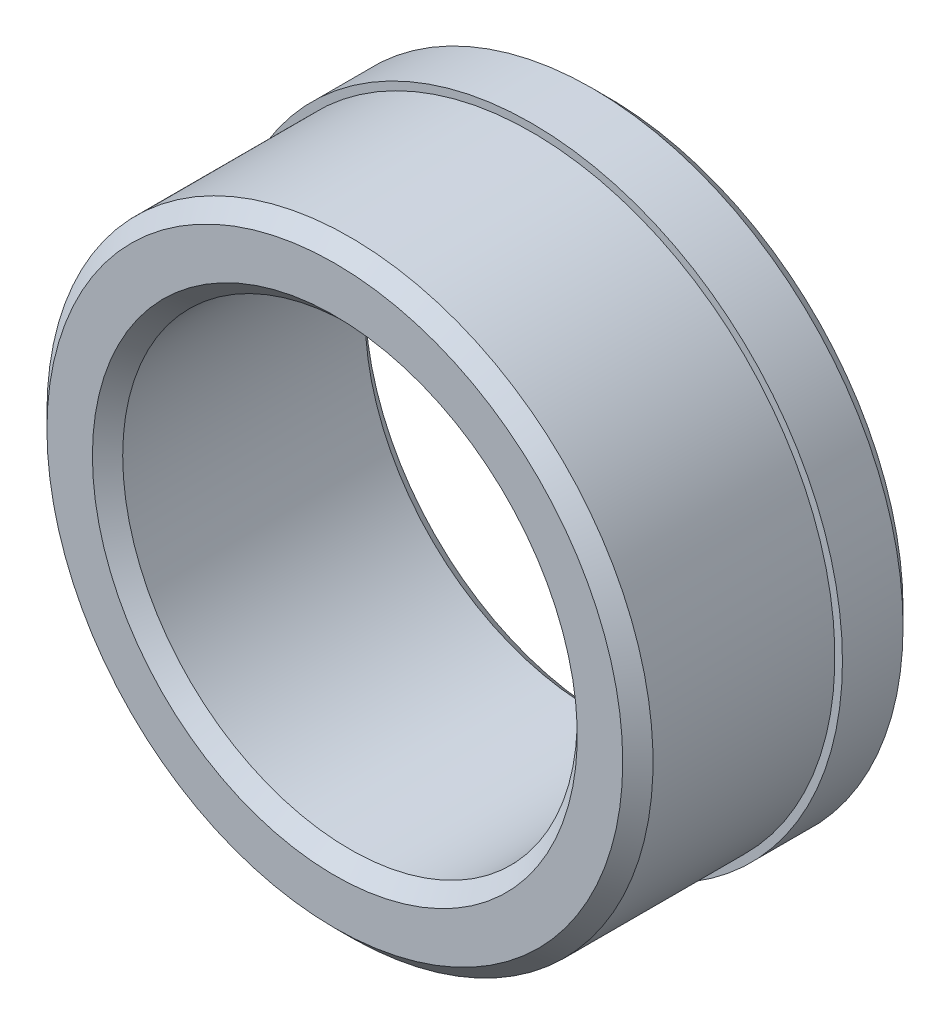
from build123d import *

# Parameters (mm, degrees)
SKETCH1_W     = 26
SKETCH1_H     = 10
SKETCH1_W_2   = 10
SKETCH1_H_2   = 1
CHAMFER1_SIZE = 2


with BuildPart() as part:
    # Sketch1 → Revolve1 (revolve)
    with BuildSketch(Plane(origin=(0, 0, 0), x_dir=(0, 0, -1), z_dir=(1, 0, 0)), mode=Mode.PRIVATE) as revolve1_sk:
        with Locations((-23, 35)):
            Rectangle(SKETCH1_W, SKETCH1_H)
        with Locations((-5, 35)):
            Rectangle(SKETCH1_W_2, SKETCH1_H)
        with Locations((-5, 40.5)):
            Rectangle(SKETCH1_W_2, SKETCH1_H_2)
    revolve(revolve1_sk.sketch.rotate(Axis((0, 0, 0), (0, 0, 1)), 90), axis=Axis((0, 0, 0), (0, 0, 1)))

    # Chamfer1
    chamfer1_edges = [part.edges().sort_by_distance(p)[0] for p in [
        (30, 0, 36),
        (40, 0, 36),
        (41, 0, 0),
        (30, 0, 0),
    ]]
    chamfer(chamfer1_edges, length=CHAMFER1_SIZE)


solid = part.part
